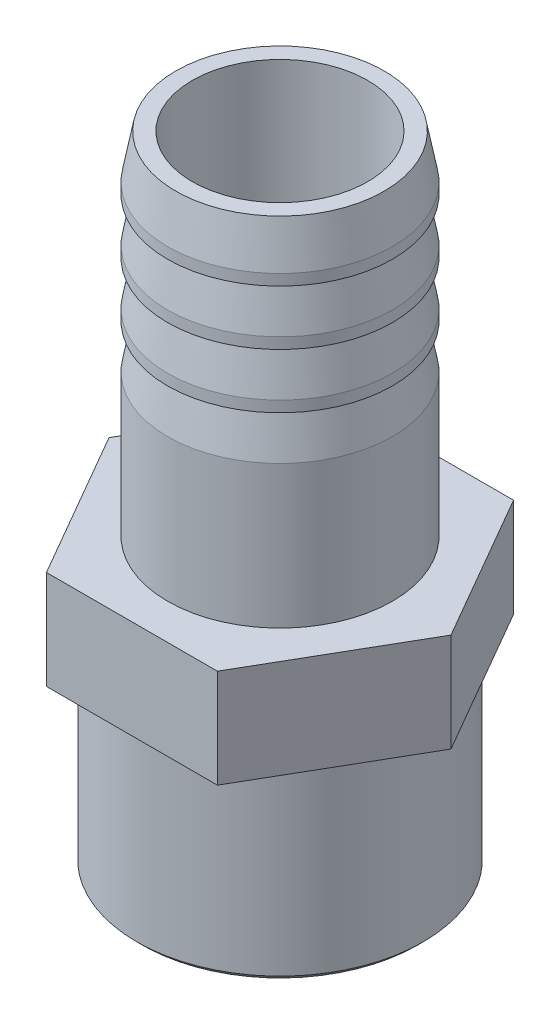
from build123d import *

# Parameters (mm, degrees)
EXTRUDE_1_DEPTH     = 9
SKETCH_3_R          = 13.05
EXTRUDE_2_DEPTH     = 17
CUT_EXTRUDE_1_REACH = 63.557
SKETCH_4_R          = 8
SKETCH_5_R          = 9
CUT_EXTRUDE_2_DEPTH = 17
CHAMFER_1_SIZE      = 0.5
CHAMFER_2_SIZE      = 0.5


with BuildPart() as part:
    # 草图1 → 旋转1 (revolve)
    with BuildSketch(Plane.XY, mode=Mode.PRIVATE) as revolve_1_sk:
        Polygon((-10.25, 13), (-9.5, 17), (-10.25, 17), (-10.25, 18), (-9.5, 22), (-10.25, 22), (-10.25, 23), (-9.5, 27), (-10.25, 27), (-10.25, 28), (-9.5, 32), (0, 32), (0, 0), (-10.25, 0), align=None)
    revolve(revolve_1_sk.sketch.rotate(Axis((0, 0, 0), (0, 1, 0)), 180), axis=Axis((0, 0, 0), (0, 1, 0)))

    # 草图2 → 凸台-拉伸1 (add)
    with BuildSketch(Plane.XZ):
        Polygon((15.588457268, 0), (7.794228634, 13.5), (-7.794228634, 13.5), (-15.588457268, 0), (-7.794228634, -13.5), (7.794228634, -13.5), align=None)
    extrude(amount=EXTRUDE_1_DEPTH)

    # 草图3 → 凸台-拉伸2 (add)
    with BuildSketch(Plane.XZ.offset(9)):
        Circle(SKETCH_3_R)
    extrude(amount=EXTRUDE_2_DEPTH)

    # 草图4 → 切除-拉伸1 (cut, up to next)
    with BuildSketch(Plane(origin=(0, 32, 0), x_dir=(1, 0, 0), z_dir=(0, 1, 0)), mode=Mode.PRIVATE) as cut_extrude_1_sk1:
        with Locations(Location((0, 0, 0), (0, 0, 180))):
            Circle(SKETCH_4_R)
    cut_extrude_1_tool1 = extrude(cut_extrude_1_sk1.sketch, amount=-CUT_EXTRUDE_1_REACH, mode=Mode.PRIVATE) & part.part
    add(cut_extrude_1_tool1.solids().sort_by_distance((0, 32, 0))[0], mode=Mode.SUBTRACT)

    # 草图5 → 切除-拉伸2 (cut)
    with BuildSketch(Plane.XZ.offset(26)):
        Circle(SKETCH_5_R)
    extrude(amount=-CUT_EXTRUDE_2_DEPTH, mode=Mode.SUBTRACT)

    # 倒角1
    chamfer_1_edges = [part.edges().sort_by_distance(p)[0] for p in [
        (-13.05, -26, 0),
    ]]
    chamfer(chamfer_1_edges, length=CHAMFER_1_SIZE)

    # 倒角2
    chamfer_2_edges = [part.edges().sort_by_distance(p)[0] for p in [
        (8, -9, 0),
    ]]
    chamfer(chamfer_2_edges, length=CHAMFER_2_SIZE)


solid = part.part
